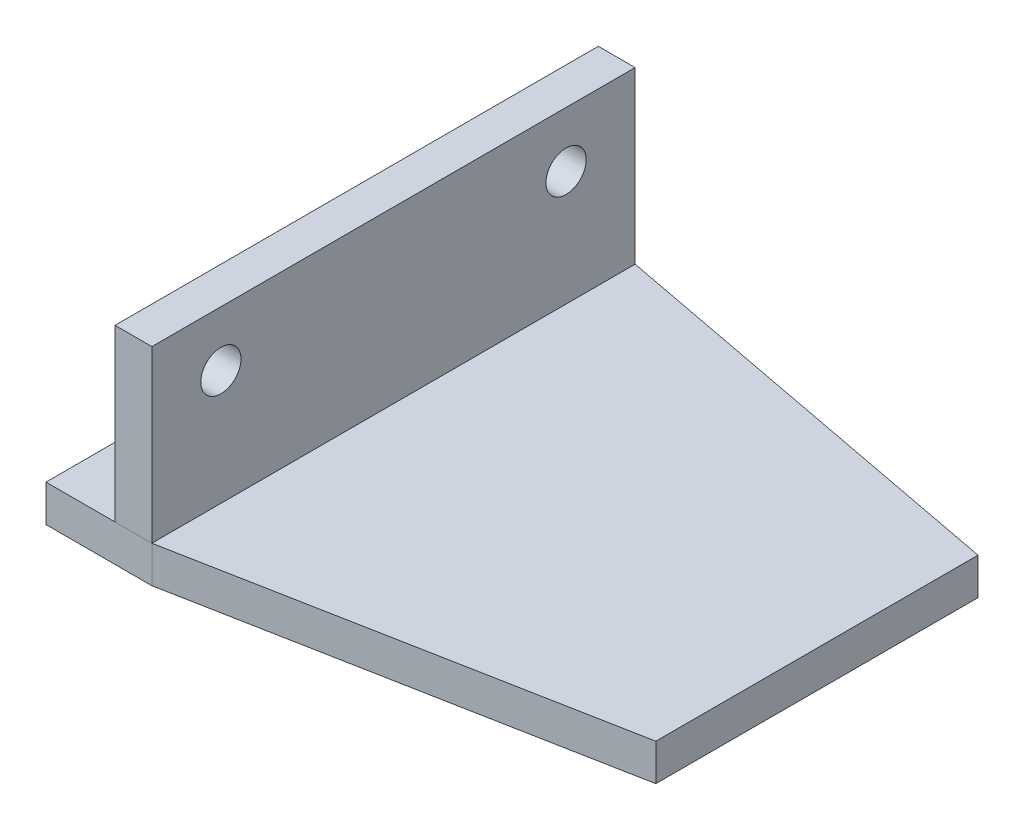
from build123d import *

# Parameters (mm, degrees)
EXTRUDE_1_DEPTH              = 16
SKETCH_2_W                   = 16
SKETCH_2_H                   = 210
EXTRUDE_2_DEPTH              = 74
HOLE_WIZARD_M20_1_AT_2_COUNT = 2
HOLE_WIZARD_M20_1_AT_2_PITCH = 150


with BuildPart() as part:
    # 草图1 → 凸台-拉伸1 (new body)
    with BuildSketch(Plane(origin=(0, 0, 0), x_dir=(1, 0, 0), z_dir=(0, 1, 0))):
        Polygon((230, -70), (230, 70), (46, 105), (0, 105), (0, -105), (46, -105), align=None)
    extrude(amount=EXTRUDE_1_DEPTH)


with BuildPart() as body_2:
    # 草图2 → 凸台-拉伸2 (new body)
    with BuildSketch(Plane(origin=(0, 16, 0), x_dir=(1, 0, 0), z_dir=(0, 1, 0))):
        with Locations((38, 0)):
            Rectangle(SKETCH_2_W, SKETCH_2_H)
    extrude(amount=EXTRUDE_2_DEPTH)

    # 草图4 → M20 螺纹孔1 (revolve, cut)
    with BuildSketch(Plane(origin=(30, 66, -75), x_dir=(0, 0, 1), z_dir=(0, 1, 0))):
        Polygon((0, 0), (0, 57.757530416), (8.75, 52.5), (8.75, 0), align=None)
    hole_wizard_m20_1 = revolve(axis=Axis((23.65, 66, -75), (1, 0, 0)), mode=Mode.SUBTRACT)

    # M20 螺纹孔1 at 2: M20 螺纹孔1 ×2
    with Locations(*[(0, 0, i * HOLE_WIZARD_M20_1_AT_2_PITCH) for i in range(1, HOLE_WIZARD_M20_1_AT_2_COUNT)]):
        add(hole_wizard_m20_1, mode=Mode.SUBTRACT)


solid = Compound([part.part, body_2.part])
